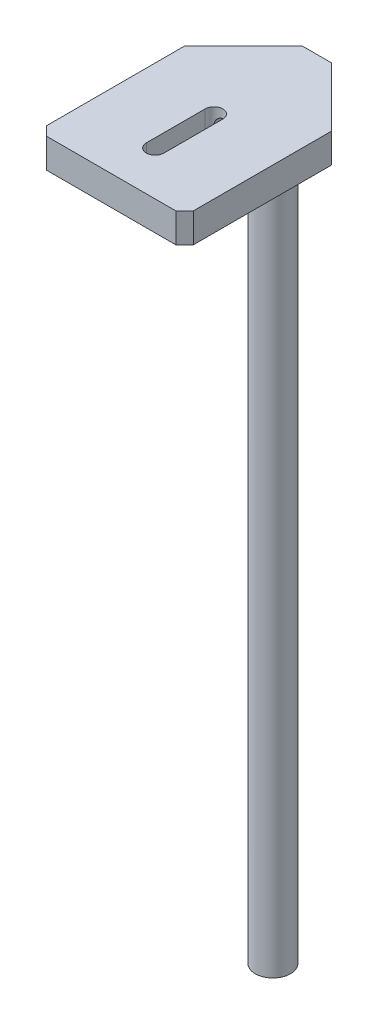
from build123d import *

# Parameters (mm, degrees)
BOSS_EXTRUDE1_DEPTH   = 10
SKETCH2_R             = 6
BOSS_EXTRUDE2_DEPTH   = 260
CUT_EXTRUDE1_DEPTH    = 256.244980362
M5_TAPPED_HOLE1_D     = 4.2
M5_TAPPED_HOLE1_DEPTH = 36.9
M5_TAPPED_HOLE1_TIP   = 1.2618073
CHAMFER1_SIZE         = 3


with BuildPart() as part:
    # Sketch1 → Boss-Extrude1 (new body)
    with BuildSketch(Plane(origin=(0, 0, 0), x_dir=(1, 0, 0), z_dir=(0, 1, 0))):
        Polygon((-25, 25), (-5, 45), (5, 45), (25, 25), (25, -25), (-25, -25), align=None)
    extrude(amount=BOSS_EXTRUDE1_DEPTH)

    # Sketch2 → Boss-Extrude2 (add)
    with BuildSketch(Plane.XZ.offset(-10)):
        with Locations(Location((0, -30, 0), (0, 0, 90))):
            Circle(SKETCH2_R)
    extrude(amount=BOSS_EXTRUDE2_DEPTH)

    # Sketch3 → Cut-Extrude1 (cut, through all)
    with BuildSketch(Plane.XZ):
        with BuildLine():
            Line((-3, -10), (-3, 10))
            ThreePointArc((-3, 10), (0, 13), (3, 10))
            Line((3, 10), (3, -10))
            ThreePointArc((3, -10), (0, -13), (-3, -10))
        make_face()
    extrude(amount=-CUT_EXTRUDE1_DEPTH, mode=Mode.SUBTRACT)

    # M5 Tapped Hole1
    with Locations(Plane(origin=(0, 0, -45), x_dir=(-1, 0, 0), z_dir=(0, 0, -1))):
        with Locations((0, 5)):
            Hole(M5_TAPPED_HOLE1_D / 2, depth=M5_TAPPED_HOLE1_DEPTH)
            with Locations((0, 0, -(M5_TAPPED_HOLE1_DEPTH + M5_TAPPED_HOLE1_TIP / 2))):  # 118° drill point
                Cone(0, M5_TAPPED_HOLE1_D / 2, M5_TAPPED_HOLE1_TIP, mode=Mode.SUBTRACT)

    # Chamfer1
    chamfer1_edges = [part.edges().sort_by_distance(p)[0] for p in [
        (25, 5, 25),
        (-25, 5, 25),
    ]]
    chamfer(chamfer1_edges, length=CHAMFER1_SIZE)


solid = part.part
